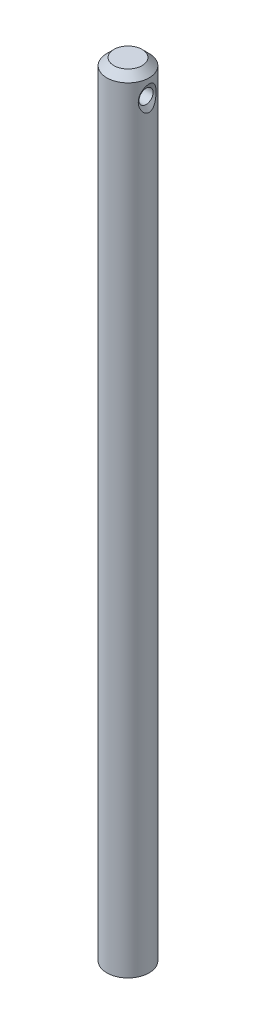
SolidWorks part; units mm, degrees
material "SS400B"
ref_plane "Front Plane" through (0, 0, 0) normal (0, 0, 1) x (1, 0, 0)
ref_plane "Top Plane" through (0, 0, 0) normal (0, 1, 0) x (1, 0, 0)
ref_plane "Right Plane" through (0, 0, 0) normal (1, 0, 0) x (0, 0, -1)
sketch "Sketch1" plane through (0, 0, 0) normal (0, 1, 0) x (1, 0, 0)
  circle A0 centre (0, 0) radius 3
  dimension "D1" = 6
extrude "Boss-Extrude1" add sketch "Sketch1" along normal blind 111
sketch "Sketch2" plane through (0, 0, 0) normal (1, 0, 0) x (0, 0, -1)
  line L0 (3, 111) -> (-3, 111) construction
  circle A0 centre (0, 107.5) radius 1
  dimension "D1" = 2
  dimension "D2" = 3.5
extrude "Cut-Extrude1" cut sketch "Sketch2" against normal through all both and the other way through all
ref_plane "Plane1" through (3, 0, 0) normal (1, 0, 0) x (0, 0, -1)
sketch "Sketch3" plane through (3, 0, 0) normal (1, 0, 0) x (0, 0, -1)
  circle A0 centre (0, 107.5) radius 1.75
  dimension "D1" = 3.5
extrude "Cut-Extrude2" cut sketch "Sketch3" against normal blind 111 draft 60
mirror "Mirror1" about plane through (0, 0, 0) normal (1, 0, 0) of "Cut-Extrude2"
chamfer "Chamfer3" distance 1 angle 45 1 edges at (0, 111, 3)
